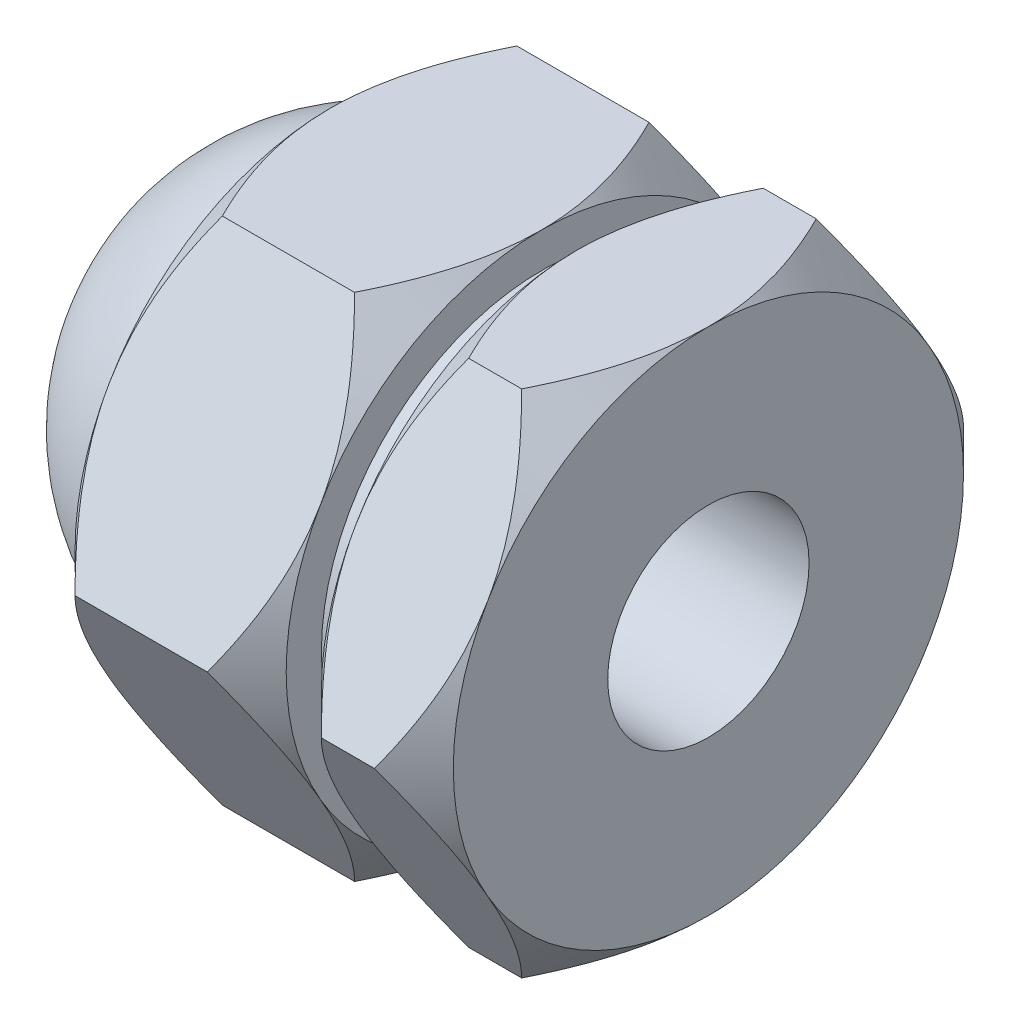
from build123d import *

# Parameters (mm, degrees)
SKETCH2_R           = 12.5
BOSS_EXTRUDE1_DEPTH = 12
SKETCH6_R           = 12.5
BOSS_EXTRUDE2_DEPTH = 7.5
SKETCH5_R           = 1
CUT_EXTRUDE2_DEPTH  = 27.750389405
CUT_EXTRUDE3_START  = -15
SKETCH7_R           = 5.7225
CUT_EXTRUDE3_DEPTH  = 15


with BuildPart() as part:
    # Sketch1 → Revolve1 (revolve)
    with BuildSketch(Plane.XY, mode=Mode.PRIVATE) as revolve1_sk:
        with BuildLine():
            Line((0, 5.7225), (0, 7.2225))
            ThreePointArc((0, 7.2225), (3.667573597, 10.968130039), (8.5, 13))
            Line((8.5, 13), (8.5, 14.5))
            Line((8.5, 14.5), (20.5, 14.5))
            Line((20.5, 14.5), (20.5, 12.5))
            Line((20.5, 12.5), (22.5, 12.5))
            Line((22.5, 12.5), (22.5, 14.5))
            Line((22.5, 14.5), (30, 14.5))
            Line((30, 14.5), (30, 0))
            Line((30, 0), (15, 0))
            Line((15, 0), (15, 5.7225))
            Line((15, 5.7225), (0, 5.7225))
        make_face()
    revolve(revolve1_sk.sketch.rotate(Axis((0, 0, 0), (1, 0, 0)), 90), axis=Axis((0, 0, 0), (1, 0, 0)))

    # Sketch2 → Boss-Extrude1 (add)
    with BuildSketch(Plane(origin=(20.5, 0, 0), x_dir=(0, 0, -1), z_dir=(1, 0, 0))):
        Polygon((16.743157806, 0), (8.371578903, 14.5), (-8.371578903, 14.5), (-16.743157806, 0), (-8.371578903, -14.5), (8.371578903, -14.5), align=None)
        with Locations(Location((0, 0, 0), (0, 0, 180))):
            Circle(SKETCH2_R, mode=Mode.SUBTRACT)
    extrude(amount=-BOSS_EXTRUDE1_DEPTH)

    # Sketch6 → Boss-Extrude2 (add)
    with BuildSketch(Plane(origin=(30, 0, 0), x_dir=(0, 0, -1), z_dir=(1, 0, 0))):
        Polygon((16.743157806, 0), (8.371578903, 14.5), (-8.371578903, 14.5), (-16.743157806, 0), (-8.371578903, -14.5), (8.371578903, -14.5), align=None)
        with Locations(Location((0, 0, 0), (0, 0, 180))):
            Circle(SKETCH6_R, mode=Mode.SUBTRACT)
    extrude(amount=-BOSS_EXTRUDE2_DEPTH)

    # Sketch3 → Cut-Revolve1 (revolve, cut)
    with BuildSketch(Plane(origin=(0, 0, 0), x_dir=(1, 0, 0), z_dir=(0, 1, 0)), mode=Mode.PRIVATE) as cut_revolve1_sk:
        Polygon((18.256842194, 16.743157806), (20.5, 14.5), (20.5, 16.743157806), align=None)
        Polygon((24.743157806, 16.743157806), (22.5, 14.5), (22.5, 16.743157806), align=None)
        Polygon((8.5, 14.5), (10.743157806, 16.743157806), (8.5, 16.743157806), align=None)
        Polygon((27.756842194, 16.743157806), (30, 16.743157806), (30, 14.5), align=None)
    revolve(cut_revolve1_sk.sketch.rotate(Axis((0, 0, 0), (-1, 0, 0)), 270), axis=Axis((0, 0, 0), (-1, 0, 0)), mode=Mode.SUBTRACT)

    # Sketch5 → Cut-Extrude2 (cut, through all)
    with BuildSketch(Plane.ZY.offset(-15)):
        Circle(SKETCH5_R)
    extrude(amount=-CUT_EXTRUDE2_DEPTH, mode=Mode.SUBTRACT)

    # Sketch7 → Cut-Extrude3 (cut)
    with BuildSketch(Plane(origin=(30, 0, 0), x_dir=(0, 0, -1), z_dir=(1, 0, 0)).offset(CUT_EXTRUDE3_START)):
        with Locations(Location((0, 0, 0), (0, 0, 180))):
            Circle(SKETCH7_R)
    extrude(amount=CUT_EXTRUDE3_DEPTH, mode=Mode.SUBTRACT)


solid = part.part
